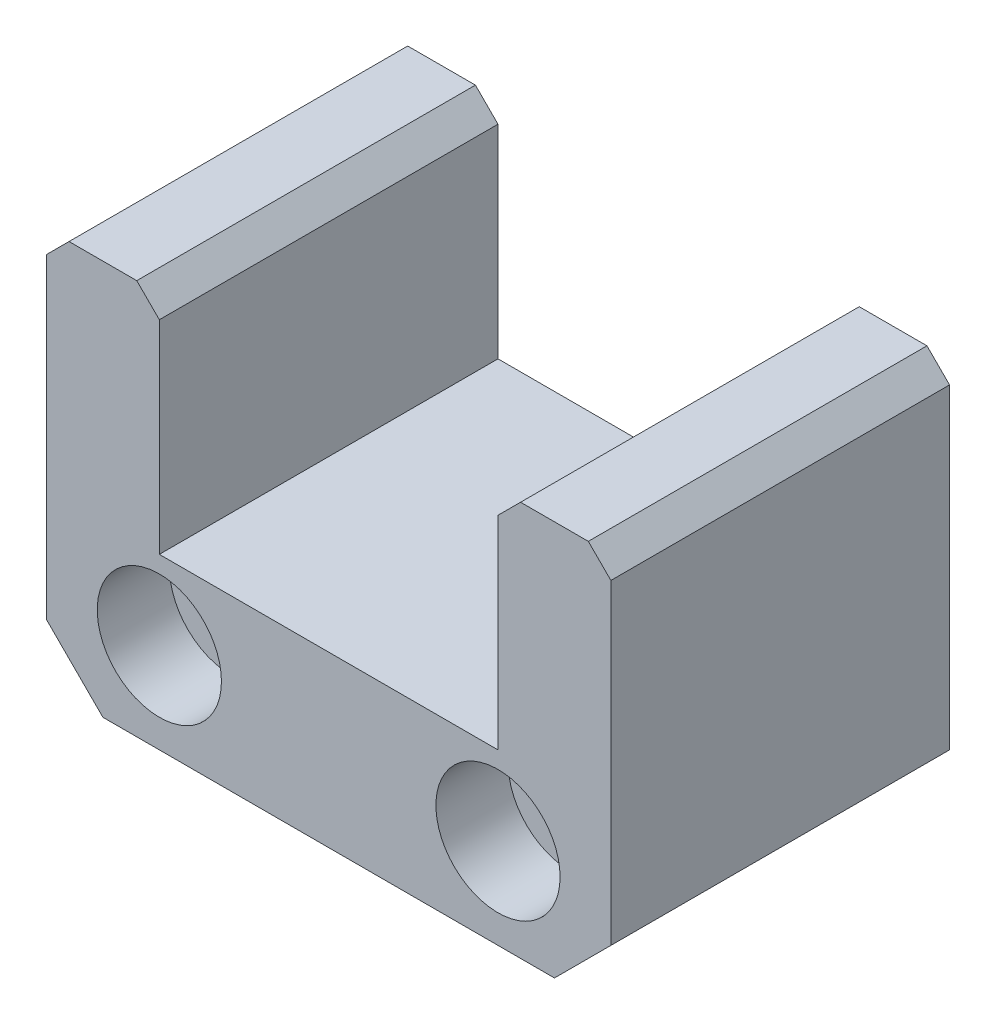
from build123d import *

# Parameters (mm, degrees)
BOSS_EXTRUDE1_DEPTH                                 = 30
CBORE_FOR_M6_HEX_SOCKET_HEAD_CAP_SCREW1_D           = 6.6
CBORE_FOR_M6_HEX_SOCKET_HEAD_CAP_SCREW1_CBORE_D     = 11
CBORE_FOR_M6_HEX_SOCKET_HEAD_CAP_SCREW1_CBORE_DEPTH = 6.4
CHAMFER1_SIZE                                       = 2
CHAMFER2_SIZE                                       = 5


with BuildPart() as part:
    # Sketch1 → Boss-Extrude1 (new body)
    with BuildSketch(Plane.XY):
        Polygon((-25, 20), (-15, 20), (-15, 0), (15, 0), (15, 20), (25, 20), (25, -15), (-25, -15), align=None)
    extrude(amount=BOSS_EXTRUDE1_DEPTH)

    # CBORE for M6 Hex Socket Head Cap Screw1 (through all)
    with Locations(Plane.XY.offset(30)):
        with Locations((-15, -7), (15, -7)):
            CounterBoreHole(CBORE_FOR_M6_HEX_SOCKET_HEAD_CAP_SCREW1_D / 2, CBORE_FOR_M6_HEX_SOCKET_HEAD_CAP_SCREW1_CBORE_D / 2, CBORE_FOR_M6_HEX_SOCKET_HEAD_CAP_SCREW1_CBORE_DEPTH)

    # Chamfer1
    chamfer1_edges = [part.edges().sort_by_distance(p)[0] for p in [
        (-25, 20, 15),
        (-15, 20, 15),
        (15, 20, 15),
        (25, 20, 15),
    ]]
    chamfer(chamfer1_edges, length=CHAMFER1_SIZE)

    # Chamfer2
    chamfer2_edges = [part.edges().sort_by_distance(p)[0] for p in [
        (25, -15, 15),
        (-25, -15, 15),
    ]]
    chamfer(chamfer2_edges, length=CHAMFER2_SIZE)


solid = part.part
